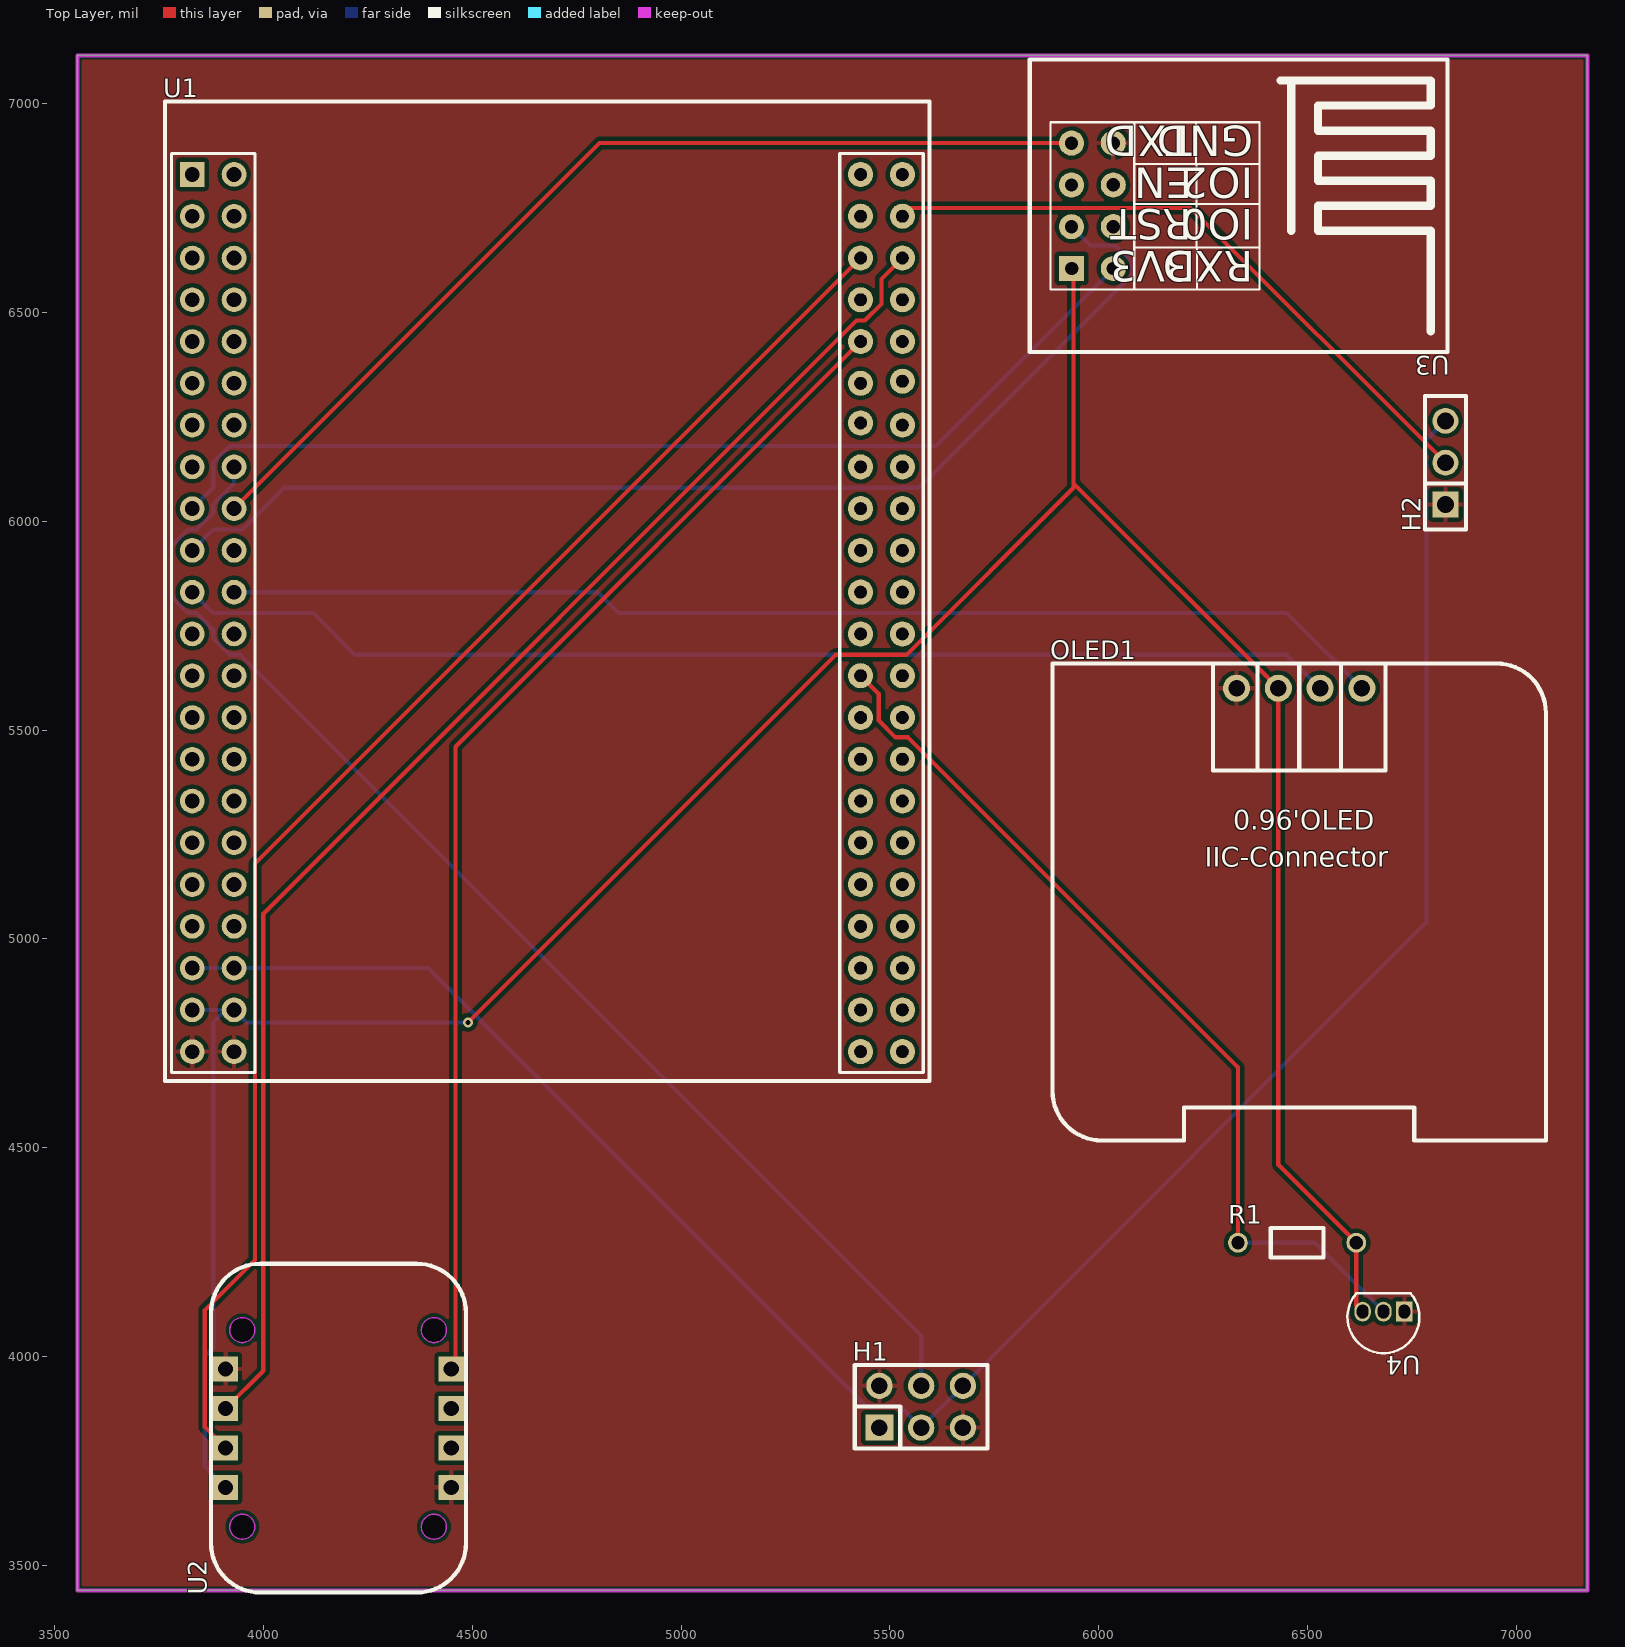
[diagram p0: Top Layer view]
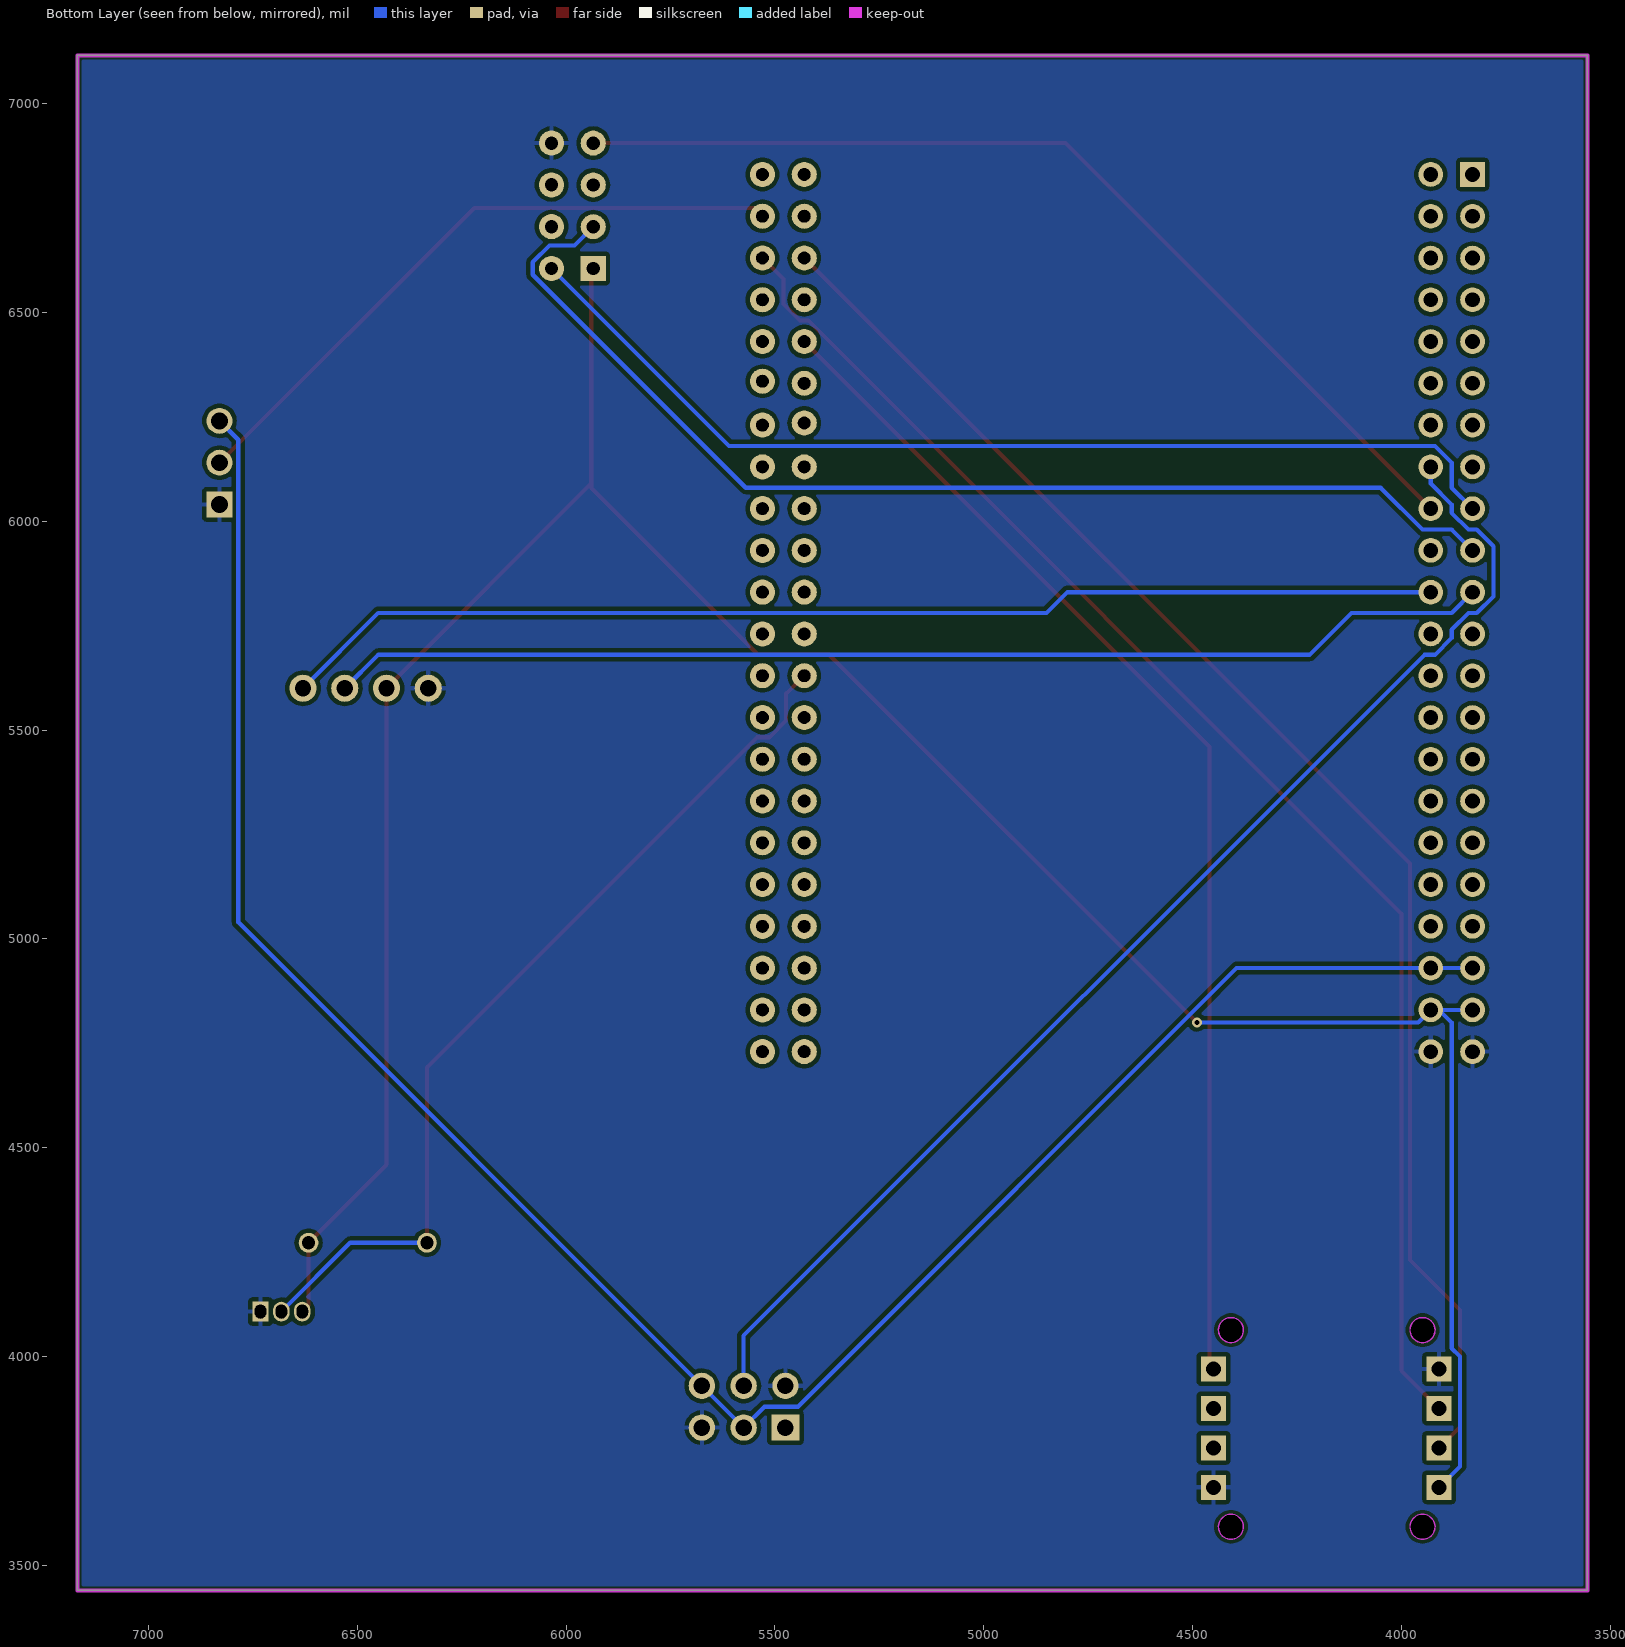
[diagram p1: Bottom Layer view, seen from below]
# Altium PCB MISC51903.pcbdoc
Units mil, origin at the board's own origin, x right, y up, seen from the top; angles counter-clockwise.
Board outline 3615 x 3675 mil, 2 copper layers (Top Layer, Bottom Layer), stack 62.206 mil thick; 8 components, 85 nets, 122 pads, 1 vias.

## Layer stack, top to bottom
Top Solder Mask Layer: solder mask 0.394, Dk 3.3
Top Layer: signal copper 1.379
Dielectric1: surface 59.449, FR4, Dk 4.5
Bottom Layer: signal copper 1.378
Bottom Solder Mask Layer: solder mask 0.394, Dk 3.3

## Board outline
3555,7115 3555,3440 7170,3440 7170,7115

## Design rules (kind name [scope] priority, off if disabled: settings)
BoardOutlineClearance copperThickness2oz_1 [All] p2 off: genericclearance=7.99 ignorepadtopadclearanceinfootprint=FALSE except(0: Arc-SplitContinuation Track-SplitContinuation SMDPad-SplitContinuation THPad-SplitContinuation Via-SplitContinuation Fill-SplitContinuation Region-SplitContinuation Poly-SplitContinuation Text-SplitContinuation Hole-SplitContinuation; 5.98: Arc-CutoutEdge SMDPad-CutoutEdge THPad-CutoutEdge Via-CutoutEdge Fill-CutoutEdge Region-CutoutEdge Text-CutoutEdge; 6.93: Hole-OutlineEdge Hole-CutoutEdge; 10: Poly-OutlineEdge Poly-CutoutEdge; 11.81: Arc-OutlineEdge Track-OutlineEdge SMDPad-OutlineEdge THPad-OutlineEdge Via-OutlineEdge Fill-OutlineEdge Region-OutlineEdge Text-OutlineEdge Track-CutoutEdge)
BoardOutlineClearance copperThickness1oz_1 [All] p4: genericclearance=4.02 ignorepadtopadclearanceinfootprint=FALSE except(0: Arc-SplitContinuation Track-SplitContinuation SMDPad-SplitContinuation THPad-SplitContinuation Via-SplitContinuation Fill-SplitContinuation Region-SplitContinuation Poly-SplitContinuation Text-SplitContinuation Hole-SplitContinuation; 6: SMDPad-CutoutEdge THPad-CutoutEdge Via-CutoutEdge Fill-CutoutEdge Region-CutoutEdge Text-CutoutEdge; 6.93: Hole-OutlineEdge Hole-CutoutEdge; 10: Poly-OutlineEdge Poly-CutoutEdge; 11.8: Arc-OutlineEdge Track-OutlineEdge SMDPad-OutlineEdge THPad-OutlineEdge Via-OutlineEdge Fill-OutlineEdge Region-OutlineEdge Text-OutlineEdge; 11.81: Arc-CutoutEdge Track-CutoutEdge)
Clearance copperThickness2oz [All] p1 off: gap=7.99 ignorepadtopadclearanceinfootprint=FALSE except(5.98: SMDPad-Track SMDPad-SMDPad THPad-Track SMDPad-THPad THPad-THPad Track-Via SMDPad-Via THPad-Via Via-Via Fill-Track Region-Track Fill-SMDPad Region-SMDPad Fill-THPad Region-THPad Fill-Via Region-Via Fill-Fill Fill-Region Region-Region Arc-Track Arc-SMDPad Arc-THPad Arc-Via Fill-Arc Region-Arc Arc-Arc Text-Track SMDPad-Text Text-THPad Text-Via Fill-Text Region-Text Arc-Text Text-Text; 6.93: Hole-Track Hole-SMDPad Hole-THPad Hole-Via Fill-Hole Region-Hole Hole-Arc Hole-Text; 10: Poly-Track Poly-SMDPad Poly-THPad Poly-Via Poly-Fill Poly-Region Poly-Poly Poly-Arc Poly-Text Poly-Hole)
Clearance copperThickness1oz [All] p3: gap=4.02 ignorepadtopadclearanceinfootprint=FALSE except(5.98: SMDPad-Track SMDPad-SMDPad THPad-Track SMDPad-THPad THPad-THPad Track-Via SMDPad-Via THPad-Via Via-Via Fill-Track Region-Track Fill-SMDPad Region-SMDPad Fill-THPad Region-THPad Fill-Via Region-Via Fill-Fill Fill-Region Region-Region; 6: Arc-Track Arc-SMDPad Arc-THPad Arc-Via Fill-Arc Region-Arc Arc-Arc Text-Track SMDPad-Text Text-THPad Text-Via Fill-Text Region-Text Arc-Text Text-Text; 6.93: Hole-Track Hole-SMDPad Hole-THPad Hole-Via Fill-Hole Region-Hole Hole-Arc Hole-Text; 10: Poly-Track Poly-SMDPad Poly-THPad Poly-Via Poly-Fill Poly-Region Poly-Poly Poly-Arc Poly-Text Poly-Hole)
Creepage creepage [All] p1: checkdistance=0 ignoreinternallayers=TRUE applytopolygonpour=TRUE
DiffPairsRouting differentialPair [All] p1: maxlimit=6 minlimit=6 mostfreqgap=6 toplayer_minwidth=5 toplayer_prefwidth=10 toplayer_maxwidth=100 toplayer_mingap=6 toplayer_prefgap=6 toplayer_maxgap=6 bottomlayer_minwidth=5 bottomlayer_prefwidth=10 bottomlayer_maxwidth=100 bottomlayer_mingap=6 bottomlayer_prefgap=6 bottomlayer_maxgap=6 maxuncoupledlength=10
HoleToHoleClearance otherClearance [All] p1: gap=11.81 allowstackedmicrovias=TRUE
Length netLength [All] p1: minlimit=0 maxlimit=0
MatchedLengths netLengthTolerance [All] p1: tolerance=1000
PasteMaskExpansion pasteMaskExpansion [All] p1: expansion=0
PlaneConnect innerPlane [All] p1: planeconnectstyle=Relief reliefexpansion=20 reliefentries=4 reliefconductorwidth=10 reliefairgap=10
PolygonConnect copperRegion [(InNet('GND'))] p1: connectstyle=Relief reliefconductorwidth=10 reliefentries=4 polygonreliefangle="90 Angle" airgapwidth=10 via.connectstyle=Relief via.reliefconductorwidth=10 via.reliefentries=4 via.polygonreliefangle="90 Angle" via.airgapwidth=10
RoutingVias viaSize [All] p1: holewidth=12.01 width=24.02 viastyle="Through Hole" minholewidth=11.81 minwidth=19.68 maxholewidth=248.03 maxwidth=393.7
SolderMaskExpansion solderMaskExpansion [IsVia] p1: expansion=-1000 istentingtop=TRUE
SolderMaskExpansion solderMaskExpansion [All] p2: expansion=2 istentingtop=FALSE
Width copperThickness2oz_2 [All] p1 off: maxlimit=100 minlimit=8 preferedwidth=10
Width copperThickness1oz_2 [All] p2: maxlimit=100 minlimit=5 preferedwidth=10

## Components (designator, comment, footprint, x,y, rotation, side; value= is the part's Value field where it differs from the comment)
H1 "" HDR-TH_6P-P2.54-V-F-R2-C3-S2.54 5575,3880 r0 top
H2 "" HDR-TH_3P-P2.54-V-F 6830,6140 r90 top
OLED1 "" 0.96OLED_4P 6480,5600 r0 top
R1 "4.7kΩ" Res_1/8W 6475,4270 r0 top
U1 "STM32F407VET6最小系统" STM32F407VET6最小系统 3760,4655 r0 top
U2 "MAX30102" MAX30102 3875,3435 r90 top
U3 "ESP01S" ESP01S 5985,6755 r180 top
U4 "DS18B20" TO-92-3_L4.5-W3.5-P1.27-L 6681.7,4107.8 r180 top

## Footprints (in the part's own frame and the unit in brackets; to place one, negate y for a bottom-side part, rotate by r counter-clockwise, add the part's x,y. Pads: shape width x height; smd on the part's side, far side on the other; paste and mask are expansions set on the pad)
0.96OLED_4P [mm]
  round 1.65 hole 1 copper offset 0,0: 1(-3.81,-0.001) 2(-1.27,0.002) 3(1.27,0.002) 4(3.81,0.002)
  silkscreen extent -15,-27.5 15,1.5
ESP01S [mil]
  rect 60x60 hole 31.89 paste+0 mask+4: 1(49.91,150.06)
  round 60 hole 31.89 paste+0 mask+4: 2(49.95,50.04) 3(49.95,-49.96) 4(49.95,-149.96) 5(-49.95,-150.06) 6(-49.95,-50.06) 7(-49.95,49.94) 8(-49.95,149.94)
  silkscreen extent -850,-350 150,350
HDR-TH_3P-P2.54-V-F [mil]
  rect 62x62 hole 40.16: 1(-100,0)
  round 62 hole 40.16: 2(0,0) 3(100,0)
  silkscreen extent -160,-49 160,49
HDR-TH_6P-P2.54-V-F-R2-C3-S2.54 [mm]
  rect 1.7x1.6 hole 1: 1(-2.54,-1.27)
  round 1.6 hole 1: 2(-2.54,1.27) 3(0,-1.27) 4(0,1.27) 5(2.54,-1.27) 6(2.54,1.27)
  silkscreen extent -4.04,-2.54 4.04,2.54
MAX30102 [mil]
  rect 60x60 hole 36: 1(251.97,-35) 2(346.46,-35) 3(440.94,-35) 4(535.43,-35) 5(251.97,-575) 6(346.46,-575) 7(440.94,-575) 8(535.43,-575)
  Board Outline Layer circle w0.1: c157.48,-74.8 r30
  Board Outline Layer circle w0.1: c157.48,-533.46 r30
  Board Outline Layer circle w0.1: c628.5,-74.8 r30
  Board Outline Layer circle w0.1: c628.5,-533.46 r30
  Board Outline Layer region: 157.48,-104.8 144.46,-101.83 134.03,-93.51 128.23,-81.48 128.23,-68.13 134.03,-56.1 144.46,-47.77 157.48,-44.8 157.48,-44.8 170.5,-47.77 180.94,-56.1 186.73,-68.13 186.73,-81.48 180.94,-93.51 170.5,-101.83 157.48,-104.8
  Board Outline Layer region: 157.48,-104.8 152.79,-104.43 148.21,-103.33 143.86,-101.53 139.85,-99.07 136.27,-96.02 133.21,-92.44 130.75,-88.42 128.95,-84.07 127.85,-79.5 127.48,-74.8 127.85,-70.11 128.95,-65.53 130.75,-61.18 133.21,-57.17 136.27,-53.59 139.85,-50.53 143.86,-48.07 148.21,-46.27 152.79,-45.17 157.48,-44.8 162.17,-45.17 166.75,-46.27 171.1,-48.07 175.11,-50.53 178.69,-53.59 181.75,-57.17 184.21,-61.18 186.01,-65.53 187.11,-70.11 187.48,-74.8 187.11,-79.5 186.01,-84.07 184.21,-88.42 181.75,-92.44 178.69,-96.02 175.11,-99.07 171.1,-101.53 166.75,-103.33 162.17,-104.43
  Board Outline Layer region: 157.48,-563.46 144.46,-560.49 134.03,-552.17 128.23,-540.14 128.23,-526.79 134.03,-514.76 144.46,-506.44 157.48,-503.46 157.48,-503.46 170.5,-506.44 180.94,-514.76 186.73,-526.79 186.73,-540.14 180.94,-552.17 170.5,-560.49 157.48,-563.46
  Board Outline Layer region: 157.48,-563.46 152.79,-563.1 148.21,-562 143.86,-560.19 139.85,-557.74 136.27,-554.68 133.21,-551.1 130.75,-547.08 128.95,-542.74 127.85,-538.16 127.48,-533.46 127.85,-528.77 128.95,-524.19 130.75,-519.84 133.21,-515.83 136.27,-512.25 139.85,-509.19 143.86,-506.73 148.21,-504.93 152.79,-503.83 157.48,-503.46 162.17,-503.83 166.75,-504.93 171.1,-506.73 175.11,-509.19 178.69,-512.25 181.75,-515.83 184.21,-519.84 186.01,-524.19 187.11,-528.77 187.48,-533.46 187.11,-538.16 186.01,-542.74 184.21,-547.08 181.75,-551.1 178.69,-554.68 175.11,-557.74 171.1,-560.19 166.75,-562 162.17,-563.1
  Board Outline Layer region: 628.5,-104.8 615.49,-101.83 605.05,-93.51 599.26,-81.48 599.26,-68.13 605.05,-56.1 615.49,-47.77 628.5,-44.8 628.5,-44.8 641.52,-47.77 651.96,-56.1 657.75,-68.13 657.75,-81.48 651.96,-93.51 641.52,-101.83 628.5,-104.8
  Board Outline Layer region: 628.5,-104.8 623.81,-104.43 619.23,-103.33 614.88,-101.53 610.87,-99.07 607.29,-96.02 604.23,-92.44 601.77,-88.42 599.97,-84.07 598.87,-79.5 598.5,-74.8 598.87,-70.11 599.97,-65.53 601.77,-61.18 604.23,-57.17 607.29,-53.59 610.87,-50.53 614.88,-48.07 619.23,-46.27 623.81,-45.17 628.5,-44.8 633.2,-45.17 637.77,-46.27 642.12,-48.07 646.14,-50.53 649.72,-53.59 652.77,-57.17 655.23,-61.18 657.04,-65.53 658.13,-70.11 658.5,-74.8 658.13,-79.5 657.04,-84.07 655.23,-88.42 652.77,-92.44 649.72,-96.02 646.14,-99.07 642.12,-101.53 637.77,-103.33 633.2,-104.43
  Board Outline Layer region: 628.5,-563.46 615.49,-560.49 605.05,-552.17 599.26,-540.14 599.26,-526.79 605.05,-514.76 615.49,-506.44 628.5,-503.46 628.5,-503.46 641.52,-506.44 651.96,-514.76 657.75,-526.79 657.75,-540.14 651.96,-552.17 641.52,-560.49 628.5,-563.46
  Board Outline Layer region: 628.5,-563.46 623.81,-563.1 619.23,-562 614.88,-560.19 610.87,-557.74 607.29,-554.68 604.23,-551.1 601.77,-547.08 599.97,-542.74 598.87,-538.16 598.5,-533.46 598.87,-528.77 599.97,-524.19 601.77,-519.84 604.23,-515.83 607.29,-512.25 610.87,-509.19 614.88,-506.73 619.23,-504.93 623.81,-503.83 628.5,-503.46 633.2,-503.83 637.77,-504.93 642.12,-506.73 646.14,-509.19 649.72,-512.25 652.77,-515.83 655.23,-519.84 657.04,-524.19 658.13,-528.77 658.5,-533.46 658.13,-538.16 657.04,-542.74 655.23,-547.08 652.77,-551.1 649.72,-554.68 646.14,-557.74 642.12,-560.19 637.77,-562 633.2,-563.1
  Multi-Layer board cut-out: 157.48,-104.8 144.46,-101.83 134.03,-93.51 128.23,-81.48 128.23,-68.13 134.03,-56.1 144.46,-47.77 157.48,-44.8 157.48,-44.8 170.5,-47.77 180.94,-56.1 186.73,-68.13 186.73,-81.48 180.94,-93.51 170.5,-101.83 157.48,-104.8
  Multi-Layer board cut-out: 157.48,-563.46 144.46,-560.49 134.03,-552.17 128.23,-540.14 128.23,-526.79 134.03,-514.76 144.46,-506.44 157.48,-503.46 157.48,-503.46 170.5,-506.44 180.94,-514.76 186.73,-526.79 186.73,-540.14 180.94,-552.17 170.5,-560.49 157.48,-563.46
  Multi-Layer board cut-out: 628.5,-104.8 615.49,-101.83 605.05,-93.51 599.26,-81.48 599.26,-68.13 605.05,-56.1 615.49,-47.77 628.5,-44.8 628.5,-44.8 641.52,-47.77 651.96,-56.1 657.75,-68.13 657.75,-81.48 651.96,-93.51 641.52,-101.83 628.5,-104.8
  Multi-Layer board cut-out: 628.5,-563.46 615.49,-560.49 605.05,-552.17 599.26,-540.14 599.26,-526.79 605.05,-514.76 615.49,-506.44 628.5,-503.46 628.5,-503.46 641.52,-506.44 651.96,-514.76 657.75,-526.79 657.75,-540.14 651.96,-552.17 641.52,-560.49 628.5,-563.46
  silkscreen extent 0,-610 787,0
Res_1/8W [mil]
  round 47.2 hole 31.5 paste+0 mask+2: 1(-141.7,2.48) 2(141.7,2.48)
  silkscreen extent -63,-33 63,38
STM32F407VET6最小系统 [mil]
  rect 59.05x59.05 hole 35.43 paste+0 mask+2: 1(70,2175)
  round 59.05 hole 35.43 paste+0 mask+2: 2(170,2175) 3(70,2075) 4(170,2075) 5(70,1975) 6(170,1975) 7(70,1875) 8(170,1875) 9(70,1775) 10(170,1775) 11(70,1675) 12(170,1675) 13(70,1575) 14(170,1575) 15(70,1475) 16(170,1475) 17(70,1375) 18(170,1375) 19(70,1275) 20(170,1275) 21(70,1175) 22(170,1175) 23(70,1075) 24(170,1075) 25(70,975) 26(170,975) 27(70,875) 28(170,875) 29(70,775) 30(170,775) 31(70,675) 32(170,675) 33(70,575) 34(170,575) 35(70,475) 36(170,475) 37(70,375) 38(170,375) 39(70,275) 40(170,275) 41(70,175) 42(170,175) 43(70,75) 44(170,75)
  round 60 hole 30 slot 30.2 at 0 deg paste+0 mask+2: 45(1770,75) 46(1670,75) 47(1770,175) 48(1670,175) 49(1770,275) 50(1670,275) 51(1770,375) 52(1670,375) 53(1770,475) 54(1670,475) 55(1770,575) 56(1670,575) 57(1770,675) 58(1670,675) 59(1770,775) 60(1670,775) 61(1770,875) 62(1670,875) 63(1770,975) 64(1670,975) 65(1770,1075) 66(1670,1075) 67(1770,1175) 68(1670,1175) 69(1770,1275) 70(1670,1275) 71(1770,1375) 72(1670,1375) 73(1770,1475) 74(1670,1475) 75(1770,1575) 76(1670,1580) 77(1770,1680) 78(1670,1675) 79(1770,1775) 80(1670,1775) 81(1770,1875) 82(1670,1875) 83(1770,1975) 84(1670,1975) 85(1770,2075) 86(1670,2075) 87(1770,2175) 88(1670,2175)
  silkscreen extent 5,5 1835,2350
TO-92-3_L4.5-W3.5-P1.27-L [mm]
  rect 1x1.2 hole 0.7 slot 0.85 at 90 deg: 1(-1.27,0)
  oval 1x1.2 hole 0.7 slot 0.85 at 90 deg: 2(0,0) 3(1.27,0)
  silkscreen extent -2.19,-1.1 2.19,2.52

## Via types
v1: diameter 24.02, hole 12, Top Layer to Bottom Layer, 1 vias

## Nets (pads, with @x,y where several pads share a name; then routed paths per layer and width w, separated by ;. In a path a pad name is that pad's centre, name@x,y a point inside that pad or via, vN(x,y) a via of type N, cw(c..) or ccw(c..) an arc to the next point about the centre after c; other vN are vias at no path point)
+5V: H1.3 H1.6 H2.3 U1.39 U1.40 | length 5130.5
  Bottom Layer w10: U1.39 U1.40 4395,4930 5445,3880 5525,3880 H1.3 H1.6 6785,5040 6785,6195 H2.3
GND: H1.2 H1.5 H2.1 OLED1.1 U1.43 U1.44 U2.4 U2.5 U3.5 U4.1
PA0: U1.15
PA1: H1.4 U1.16 | length 3043.7
  Bottom Layer w10: U1.16 3930,6090 3880,6040 3880,6020 3840,5980 3820,5980 3780,5940 3780,5820 3820,5780 3840,5780 3880,5740 3880,5720 3920,5680 3945,5680 5575,4050 H1.4
PA2: U1.17 U3.8 | length 2478.3
  Bottom Layer w10: U1.17 3880,6080 3880,6140 3920,6180 5609.89,6180 U3.8@6034.95,6605.06
PA3: U1.18 U3.4 | length 2367.5
  Top Layer w10: U1.18 4804.96,6904.96 U3.4
PA4: U1.19 U3.2 | length 2733.6
  Bottom Layer w10: U1.19 3880,5980 3950,5980 4050,6080 5570,6080 6079.99,6590 6079.99,6620 6039.99,6660 5979.87,6660 U3.2
PA5: U1.20
PA6: OLED1.3 U1.21 | length 2795.3
  Bottom Layer w10: U1.21 3879.95,5780.05 4120.01,5780.05 4220.01,5680.05 6450,5680.05 OLED1.3
PA7: OLED1.4 U1.22 | length 2795.3
  Bottom Layer w10: U1.22 4800.06,5830 4850,5780.05 6450,5780.05 OLED1.4
PA8: U1.61
PA9: U1.62
PA10: U1.63
PA11: R1.1 U1.64 U4.2 | length 2165.9
  Top Layer w10: U1.64 5473.3,5586.69 5473.3,5522.47 5513.3,5482.47 5543.3,5482.47 6333.3,4692.47 R1.1
  Bottom Layer w10: R1.1 6517.03,4272.48 U4.2
PA12: U1.65
PA13: U1.66
PA14: U1.67
PA15: U1.68
PB0: U1.25
PB1: U1.26
PB2: U1.27
PB3: U1.80 U2.8 | length 2865.5
  Top Layer w10: U2.8 4460,3980.44 4460,5460 U1.80
PB4: U1.81
PB5: U1.82
PB6: U1.83 U2.3 | length 3436.8
  Top Layer w10: U2.3 4000,3965.95 4000,5060 5420,6480 5440,6480 5480,6520 5480,6580 U1.83
PB7: U1.84 U2.2 | length 3519.6
  Top Layer w10: U2.2 3860,3831.45 3860,4111.34 3980,4231.34 3980,5180 U1.84
PB8: H2.2 U1.85 | length 1561
  Top Layer w10: U1.85 5550,6750 6220,6750 H2.2
PB9: U1.86
PB10: U1.37
PB11: U1.38
PB12: U1.45
PB13: U1.46
PB14: U1.47
PB15: U1.48
PC0: U1.11
PC1: U1.12
PC2: U1.13
PC3: U1.14
PC4: U1.23
PC5: U1.24
PC6: U1.57
PC7: U1.58
PC8: U1.59
PC9: U1.60
PC10: U1.69
PC11: U1.70
PC12: U1.71
PC13: U1.7
PC14: U1.8
PC15: U1.9
PD0: U1.72
PD1: U1.73
PD2: U1.74
PD3: U1.75
PD4: U1.76
PD5: U1.77
PD6: U1.78
PD7: U1.79
PD8: U1.49
PD9: U1.50
PD10: U1.51
PD11: U1.52
PD12: U1.53
PD13: U1.54
PD14: U1.55
PD15: U1.56
PE0: U1.87
PE1: U1.88
PE2: U1.1
PE3: U1.2
PE4: U1.3
PE5: U1.4
PE6: U1.5
PE7: U1.28
PE8: U1.29
PE9: U1.30
PE10: U1.31
PE11: U1.32
PE12: U1.33
PE13: U1.34
PE14: U1.35
PE15: U1.36
RST: U1.10
VBAT: U1.6
VCC: OLED1.2 R1.2 U1.41 U1.42 U2.1 U3.1 U4.3 | length 6632.7
  Top Layer w10: v1(4490.01,4800.05) 5370,5680.05 5540,5680.05 5940,6080.05 5940,6090.05 ; U3.1 5940,6600.03 5940,6090.05 ; U4.3 6616.7,4122.81 R1.2 6430,4459.18 OLED1.2 5940,6090.05
  Bottom Layer w10: U1.41 U1.42@3910,4830 ; U2.1 3860,3736.97 3860,4000 3880,4020 3880,4800 U1.42@3910,4830 ; v1(4490.01,4800.05) 3959.94,4800.05 U1.42 U1.42@3910,4830
pads on no net: H1.1 U2.6 U2.7 U3.3 U3.6 U3.7

## Polygon pours and split planes (outlines as drawn)
GND on Top Layer (solid, remove dead copper, pour order 0): 3015,7380 3015,3095 7720,3095 7720,7380
GND on Bottom Layer (solid, remove dead copper, pour order 2): 3000,7395 3000,3000 7755,3000 7755,7395

## Keep-outs
Board Outline Layer:
  the board outline again, w10